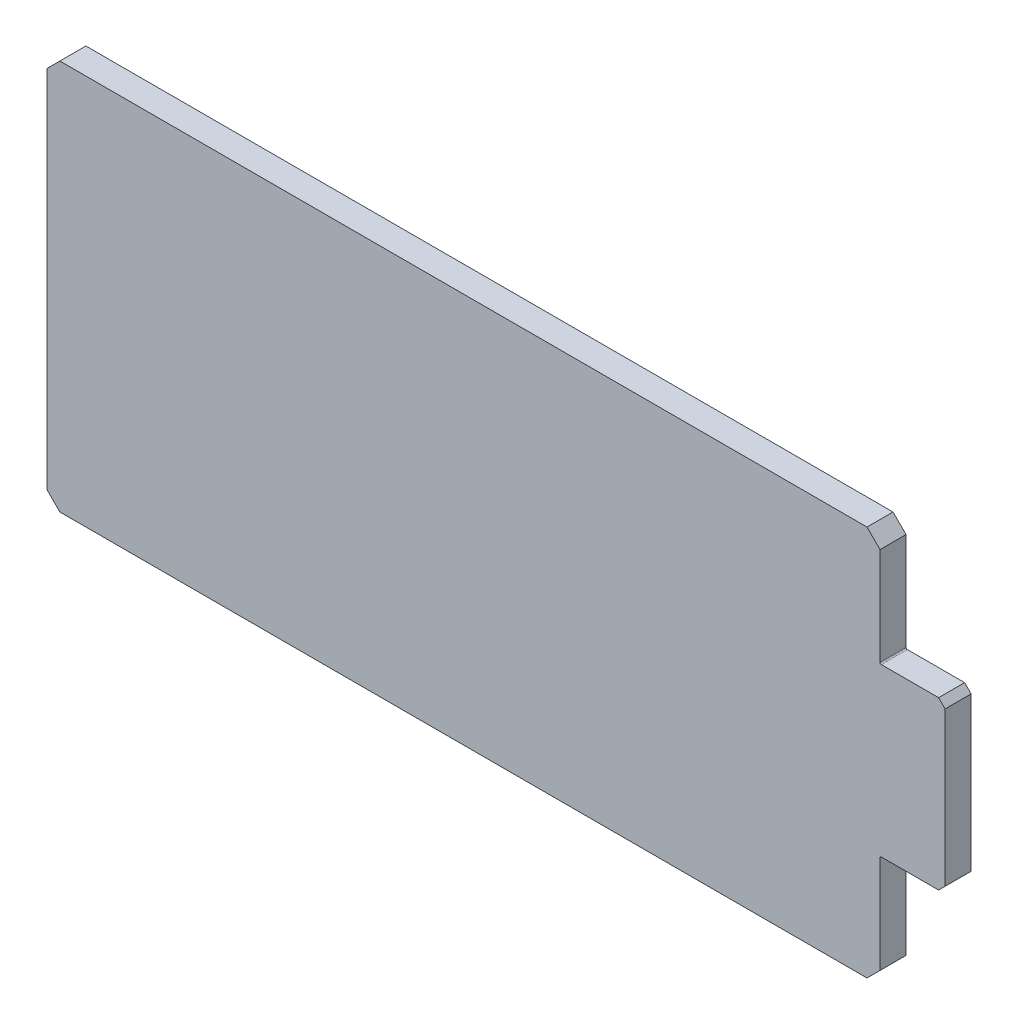
SolidWorks part; units mm, degrees
ref_plane "Front Plane" through (0, 0, 0) normal (0, 0, 1) x (1, 0, 0)
ref_plane "Top Plane" through (0, 0, 0) normal (0, 1, 0) x (1, 0, 0)
ref_plane "Right Plane" through (0, 0, 0) normal (1, 0, 0) x (0, 0, -1)
sketch "Sketch1" plane through (0, 0, 0) normal (0, 0, 1) x (1, 0, 0)
  line L0 (-58.7413, 0) -> (676.4506, 0) construction
  line L1 (-38.7707, -150) -> (-38.7707, 150)
  line L2 (-38.7707, 150) -> (601.2293, 150)
  line L3 (601.2293, 150) -> (601.2293, 64)
  line L4 (601.2293, 64) -> (651.2293, 64)
  line L5 (651.2293, 64) -> (651.2293, -64)
  line L6 (601.2293, -150) -> (601.2293, -64)
  line L7 (601.2293, -64) -> (651.2293, -64)
  line L8 (-38.7707, -150) -> (601.2293, -150)
  point P10 (651.2293, 0)
  point P13 (-38.7707, 0)
extrude "Boss-Extrude1" add sketch "Sketch1" along normal blind 20
chamfer "Chamfer1" distance 10 angle 45 4 edges at (601.2293, 150, 10) (601.2293, -150, 10) (-38.7707, -150, 10) (-38.7707, 150, 10)
fillet "Fillet1" radius 1 2 edges at (601.2293, 64, 10) (601.2293, -64, 10)
chamfer "Chamfer2" distance 5 angle 45 2 edges at (651.2293, -64, 10) (651.2293, 64, 10)
